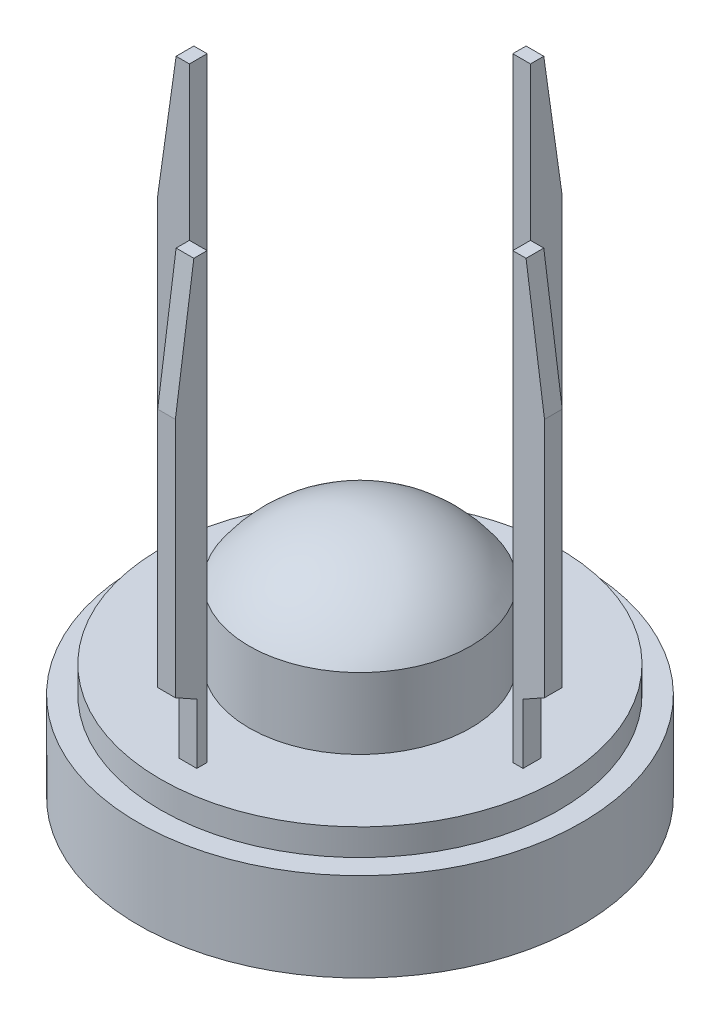
SolidWorks part; units mm, degrees
ref_plane "Front Plane" through (0, 0, 0) normal (0, 0, 1) x (1, 0, 0)
ref_plane "Top Plane" through (0, 0, 0) normal (0, 1, 0) x (1, 0, 0)
ref_plane "Right Plane" through (0, 0, 0) normal (1, 0, 0) x (0, 0, -1)
sketch "Sketch1" plane through (0, 0, 0) normal (0, 0, 1) x (1, 0, 0)
  line L0 (0, 0) -> (0, 100)
  line L1 (0, 100) -> (250, 100)
  line L2 (250, 100) -> (250, 0)
  line L3 (250, 0) -> (0, 0)
  dimension "D1" = 250
  dimension "D2" = 100
revolve "Revolve1" add sketch "Sketch1" angle 360 about L0
sketch "Sketch2" plane through (0, 100, 0) normal (0, 1, 0) x (1, 0, 0)
  circle A0 centre (0, 0) radius 225
  dimension "D1" = 450
extrude "Boss-Extrude1" add sketch "Sketch2" along normal blind 30
sketch "Sketch3" plane through (0, 130, 0) normal (0, 1, 0) x (1, 0, 0)
  circle A0 centre (0, 0) radius 125
  dimension "D1" = 250
extrude "Boss-Extrude2" add sketch "Sketch3" along normal blind 80
sketch "Sketch4" plane through (0, 0, 0) normal (0, 0, 1) x (1, 0, 0)
  line L0 (0, 210) -> (0, 275.5188)
  line L1 (125, 210) -> (-125, 210) construction
  line L2 (0, 210) -> (125, 210)
  arc A0 (125, 210) -> (0, 275.5188) centre (0, 123.5188) ccw
  dimension "D1" = 152
revolve "Revolve2" add sketch "Sketch4" angle 360 about L0
sketch "Sketch5" plane through (0, 0, 0) normal (0, 0, 1) x (1, 0, 0)
  line L0 (225, 130) -> (-225, 130) construction
  line L1 (-194.0034, 130) -> (-182.3583, 130)
  line L2 (-194.0034, 130) -> (-194.0034, 197.6873)
  line L4 (-182.3583, 130) -> (-182.3583, 145.2629)
  line L5 (-182.3583, 145.2629) -> (-182.3583, 630)
  line L6 (-182.3583, 630) -> (-197.3653, 630)
  line L7 (-197.3653, 630) -> (-218.1618, 483.0585)
  line L8 (-218.1618, 483.0585) -> (-218.1618, 211.1019)
  line L9 (-218.1618, 211.1019) -> (-194.0034, 197.6873)
  dimension "D1" = 500
extrude "Boss-Extrude3" add sketch "Sketch5" along normal mid plane 20
pattern_circular "CirPattern1" count 4 over 360 about axis through (0, 0, 0) along (0, 1, 0) of "Boss-Extrude3"
